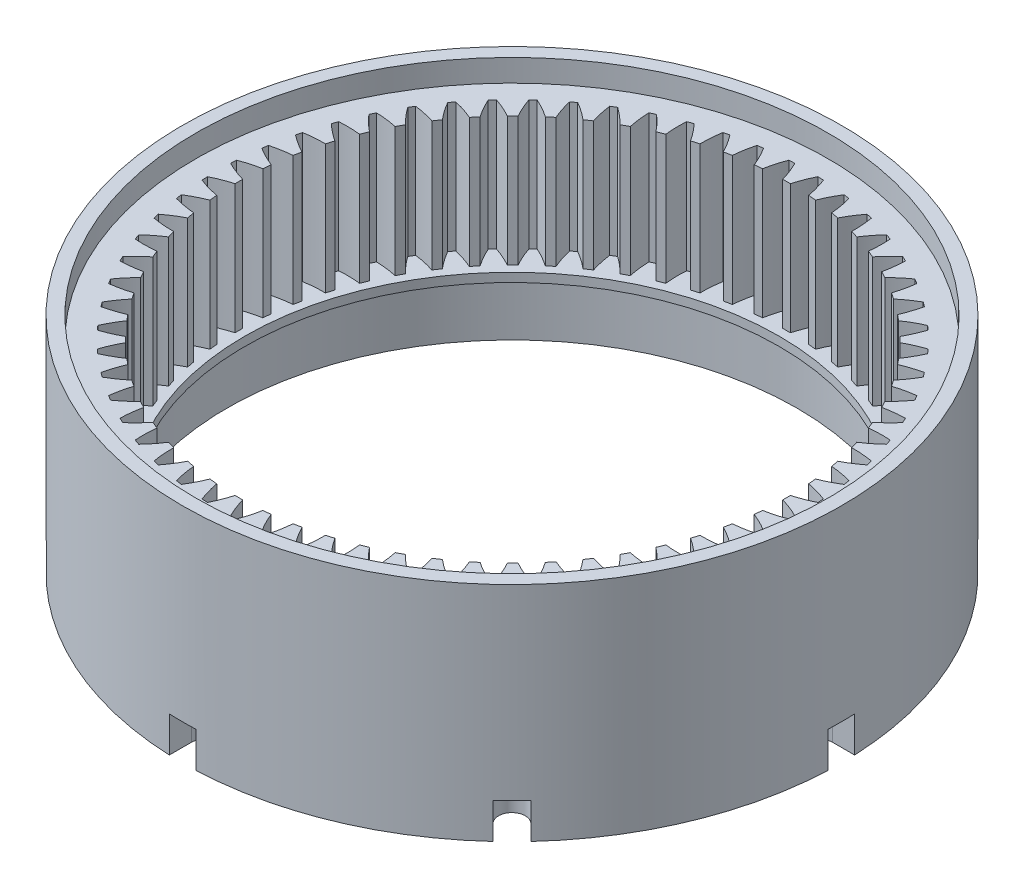
SolidWorks part; units mm, degrees
ref_plane "Front Plane" through (0, 0, 0) normal (0, 0, 1) x (1, 0, 0)
ref_plane "Top Plane" through (0, 0, 0) normal (0, 1, 0) x (1, 0, 0)
ref_plane "Right Plane" through (0, 0, 0) normal (1, 0, 0) x (0, 0, -1)
other "Configuration Table"
sketch "Sketch1" plane through (0, 0, 0) normal (0, 1, 0) x (1, 0, 0)
  circle A0 centre (0, 0) radius 37
  dimension "D1" = 74
extrude "Boss-Extrude1" add sketch "Sketch1" along normal blind 25
sketch "Sketch2" plane through (0, 25, 0) normal (0, 1, 0) x (1, 0, 0)
  circle A0 centre (0, 0) radius 35.5
  dimension "D1" = 71
extrude "Cut-Extrude1" cut sketch "Sketch2" against normal blind 2.5
sketch "Sketch3" plane through (0, 22.5, 0) normal (0, 1, 0) x (1, 0, 0)
  arc A3 (-33.0981, 1.5008) -> (-30.8696, 0.6337) centre (-27.3625, 12.9438) ccw
  arc A4 (-30.8696, 0.6337) -> (-30.8696, -0.2219) centre (-0.1235, 0.2059) ccw
  arc A5 (-30.8696, -0.2219) -> (-33.0981, -1.0891) centre (-27.3625, -12.5321) ccw
  arc A6 (-33.0981, -1.0891) -> (-33.0663, -1.7375) centre (-0.1235, 0.2059) ccw
  arc A7 (-33.0663, -1.7375) -> (-30.7634, -2.382) centre (-28.4798, 10.2126) ccw
  arc A8 (-30.7634, -2.382) -> (-30.6796, -3.2335) centre (-0.1235, 0.2059) ccw
  arc A9 (-30.6796, -3.2335) -> (-32.8124, -4.3149) centre (-25.9828, -15.1406) ccw
  arc A10 (-32.8124, -4.3149) -> (-32.7172, -4.9571) centre (-0.1235, 0.2059) ccw
  arc A11 (-32.7172, -4.9571) -> (-30.3622, -5.3728) centre (-29.3241, 7.385) ccw
  arc A12 (-30.3622, -5.3728) -> (-30.1953, -6.2119) centre (-0.1235, 0.2059) ccw
  arc A13 (-30.1953, -6.2119) -> (-32.2119, -7.4972) centre (-24.354, -17.6013) ccw
  arc A14 (-32.2119, -7.4972) -> (-32.0541, -8.1269) centre (-0.1235, 0.2059) ccw
  arc A15 (-32.0541, -8.1269) -> (-29.6698, -8.3099) centre (-29.8872, 4.4883) ccw
  arc A16 (-29.6698, -8.3099) -> (-29.4215, -9.1286) centre (-0.1235, 0.2059) ccw
  arc A17 (-29.4215, -9.1286) -> (-31.3023, -10.6053) centre (-22.4919, -19.8906) ccw
  arc A18 (-31.3023, -10.6053) -> (-31.0836, -11.2166) centre (-0.1235, 0.2059) ccw
  arc A19 (-31.0836, -11.2166) -> (-28.6929, -11.1649) centre (-30.1636, 1.5503) ccw
  arc A20 (-28.6929, -11.1649) -> (-28.3655, -11.9553) centre (-0.1235, 0.2059) ccw
  arc A21 (-28.3655, -11.9553) -> (-30.0925, -13.6093) centre (-20.4144, -21.9863) ccw
  arc A22 (-30.0925, -13.6093) -> (-29.815, -14.1962) centre (-0.1235, 0.2059) ccw
  arc A23 (-29.815, -14.1962) -> (-27.4408, -13.9104) centre (-30.1508, -1.4006) ccw
  arc A24 (-27.4408, -13.9104) -> (-27.0375, -14.6649) centre (-0.1235, 0.2059) ccw
  arc A25 (-27.0375, -14.6649) -> (-28.5941, -16.4803) centre (-18.1415, -23.8683) ccw
  arc A26 (-28.5941, -16.4803) -> (-28.2603, -17.0371) centre (-0.1235, 0.2059) ccw
  arc A27 (-28.2603, -17.0371) -> (-25.9256, -16.52) centre (-29.8487, -4.336) ccw
  arc A28 (-25.9256, -16.52) -> (-25.4503, -17.2314) centre (-0.1235, 0.2059) ccw
  arc A29 (-25.4503, -17.2314) -> (-26.8215, -19.1905) centre (-15.6951, -25.5185) ccw
  arc A30 (-26.8215, -19.1905) -> (-26.4347, -19.712) centre (-0.1235, 0.2059) ccw
  arc A31 (-26.4347, -19.712) -> (-24.1619, -18.9685) centre (-29.2604, -7.2277) ccw
  arc A32 (-24.1619, -18.9685) -> (-23.6192, -19.6299) centre (-0.1235, 0.2059) ccw
  arc A33 (-23.6192, -19.6299) -> (-24.7917, -21.714) centre (-13.0986, -26.9209) ccw
  arc A34 (-24.7917, -21.714) -> (-24.3557, -22.195) centre (-0.1235, 0.2059) ccw
  arc A35 (-24.3557, -22.195) -> (-22.1667, -21.2323) centre (-28.3915, -10.0479) ccw
  arc A36 (-22.1667, -21.2323) -> (-21.5618, -21.8373) centre (-0.1235, 0.2059) ccw
  arc A37 (-21.5618, -21.8373) -> (-22.5244, -24.0263) centre (-10.3773, -28.062) ccw
  arc A38 (-22.5244, -24.0263) -> (-22.0434, -24.4623) centre (-0.1235, 0.2059) ccw
  arc A39 (-22.0434, -24.4623) -> (-19.9593, -23.2897) centre (-27.2503, -12.7692) ccw
  arc A40 (-19.9593, -23.2897) -> (-19.2979, -23.8325) centre (-0.1235, 0.2059) ccw
  arc A41 (-19.2979, -23.8325) -> (-20.0414, -26.1053) centre (-7.5572, -28.931) ccw
  arc A42 (-20.0414, -26.1053) -> (-19.5199, -26.492) centre (-0.1235, 0.2059) ccw
  arc A43 (-19.5199, -26.492) -> (-17.5608, -25.1208) centre (-25.8479, -15.3656) ccw
  arc A44 (-17.5608, -25.1208) -> (-16.8494, -25.5962) centre (-0.1235, 0.2059) ccw
  arc A45 (-16.8494, -25.5962) -> (-17.3665, -27.9309) centre (-4.6655, -29.5193) ccw
  arc A46 (-17.3665, -27.9309) -> (-16.8097, -28.2647) centre (-0.1235, 0.2059) ccw
  arc A47 (-16.8097, -28.2647) -> (-14.9944, -26.708) centre (-24.1977, -17.8121) ccw
  arc A48 (-14.9944, -26.708) -> (-14.2398, -27.1113) centre (-0.1235, 0.2059) ccw
  arc A49 (-14.2398, -27.1113) -> (-14.5256, -29.4855) centre (-1.73, -29.8213) ccw
  arc A50 (-14.5256, -29.4855) -> (-13.9387, -29.7631) centre (-0.1235, 0.2059) ccw
  arc A51 (-13.9387, -29.7631) -> (-12.2847, -28.036) centre (-22.3158, -20.085) ccw
  arc A52 (-12.2847, -28.036) -> (-11.4943, -28.3634) centre (-0.1235, 0.2059) ccw
  arc A53 (-11.4943, -28.3634) -> (-11.546, -30.7542) centre (1.2209, -29.8342) ccw
  arc A54 (-11.546, -30.7542) -> (-10.9347, -30.9729) centre (-0.1235, 0.2059) ccw
  arc A55 (-10.9347, -30.9729) -> (-9.458, -29.092) centre (-20.22, -22.1625) ccw
  arc A56 (-9.458, -29.092) -> (-8.6393, -29.3404) centre (-0.1235, 0.2059) ccw
  arc A57 (-8.6393, -29.3404) -> (-8.4564, -31.7247) centre (4.1589, -29.5578) ccw
  arc A58 (-8.4564, -31.7247) -> (-7.8266, -31.8825) centre (-0.1235, 0.2059) ccw
  arc A59 (-7.8266, -31.8825) -> (-6.5413, -29.8659) centre (-17.9308, -24.0246) ccw
  arc A60 (-6.5413, -29.8659) -> (-5.7022, -30.0328) centre (-0.1235, 0.2059) ccw
  arc A61 (-5.7022, -30.0328) -> (-5.2865, -32.3877) centre (7.0556, -28.9947) ccw
  arc A62 (-5.2865, -32.3877) -> (-4.6443, -32.483) centre (-0.1235, 0.2059) ccw
  arc A63 (-4.6443, -32.483) -> (-3.5629, -30.3502) centre (-15.47, -25.6533) ccw
  arc A64 (-3.5629, -30.3502) -> (-2.7115, -30.434) centre (-0.1235, 0.2059) ccw
  arc A65 (-2.7115, -30.434) -> (-2.0669, -32.7368) centre (9.8832, -28.1504) ccw
  arc A66 (-2.0669, -32.7368) -> (-1.4185, -32.7687) centre (-0.1235, 0.2059) ccw
  arc A67 (-1.4185, -32.7687) -> (-0.5513, -30.5401) centre (-12.8615, -27.033) ccw
  arc A68 (-0.5513, -30.5401) -> (0.3042, -30.5401) centre (-0.1235, 0.2059) ccw
  arc A69 (0.3042, -30.5401) -> (1.1714, -32.7687) centre (12.6144, -27.033) ccw
  arc A70 (1.1714, -32.7687) -> (1.8198, -32.7368) centre (-0.1235, 0.2059) ccw
  arc A71 (1.8198, -32.7368) -> (2.4644, -30.434) centre (-10.1303, -28.1504) ccw
  arc A72 (2.4644, -30.434) -> (3.3158, -30.3502) centre (-0.1235, 0.2059) ccw
  arc A73 (3.3158, -30.3502) -> (4.3972, -32.483) centre (15.223, -25.6533) ccw
  arc A74 (4.3972, -32.483) -> (5.0394, -32.3877) centre (-0.1235, 0.2059) ccw
  arc A75 (5.0394, -32.3877) -> (5.4552, -30.0328) centre (-7.3027, -28.9947) ccw
  arc A76 (5.4552, -30.0328) -> (6.2943, -29.8659) centre (-0.1235, 0.2059) ccw
  arc A77 (6.2943, -29.8659) -> (7.5795, -31.8825) centre (17.6837, -24.0246) ccw
  arc A78 (7.5795, -31.8825) -> (8.2093, -31.7247) centre (-0.1235, 0.2059) ccw
  arc A79 (8.2093, -31.7247) -> (8.3922, -29.3404) centre (-4.4059, -29.5578) ccw
  arc A80 (8.3922, -29.3404) -> (9.2109, -29.092) centre (-0.1235, 0.2059) ccw
  arc A81 (9.2109, -29.092) -> (10.6877, -30.9729) centre (19.973, -22.1625) ccw
  arc A82 (10.6877, -30.9729) -> (11.2989, -30.7542) centre (-0.1235, 0.2059) ccw
  arc A83 (11.2989, -30.7542) -> (11.2472, -28.3634) centre (-1.468, -29.8342) ccw
  arc A84 (11.2472, -28.3634) -> (12.0377, -28.036) centre (-0.1235, 0.2059) ccw
  arc A85 (12.0377, -28.036) -> (13.6917, -29.7631) centre (22.0687, -20.085) ccw
  arc A86 (13.6917, -29.7631) -> (14.2785, -29.4855) centre (-0.1235, 0.2059) ccw
  arc A87 (14.2785, -29.4855) -> (13.9928, -27.1113) centre (1.4829, -29.8213) ccw
  arc A88 (13.9928, -27.1113) -> (14.7473, -26.708) centre (-0.1235, 0.2059) ccw
  arc A89 (14.7473, -26.708) -> (16.5626, -28.2647) centre (23.9507, -17.8121) ccw
  arc A90 (16.5626, -28.2647) -> (17.1195, -27.9309) centre (-0.1235, 0.2059) ccw
  arc A91 (17.1195, -27.9309) -> (16.6024, -25.5962) centre (4.4184, -29.5193) ccw
  arc A92 (16.6024, -25.5962) -> (17.3137, -25.1208) centre (-0.1235, 0.2059) ccw
  arc A93 (17.3137, -25.1208) -> (19.2729, -26.492) centre (25.6008, -15.3656) ccw
  arc A94 (19.2729, -26.492) -> (19.7943, -26.1053) centre (-0.1235, 0.2059) ccw
  arc A95 (19.7943, -26.1053) -> (19.0509, -23.8325) centre (7.3101, -28.931) ccw
  arc A96 (19.0509, -23.8325) -> (19.7122, -23.2897) centre (-0.1235, 0.2059) ccw
  arc A97 (19.7122, -23.2897) -> (21.7963, -24.4623) centre (27.0032, -12.7692) ccw
  arc A98 (21.7963, -24.4623) -> (22.2774, -24.0263) centre (-0.1235, 0.2059) ccw
  arc A99 (22.2774, -24.0263) -> (21.3147, -21.8373) centre (10.1302, -28.062) ccw
  arc A100 (21.3147, -21.8373) -> (21.9197, -21.2323) centre (-0.1235, 0.2059) ccw
  arc A101 (21.9197, -21.2323) -> (24.1087, -22.195) centre (28.1444, -10.0479) ccw
  arc A102 (24.1087, -22.195) -> (24.5447, -21.714) centre (-0.1235, 0.2059) ccw
  arc A103 (24.5447, -21.714) -> (23.3721, -19.6299) centre (12.8516, -26.9209) ccw
  arc A104 (23.3721, -19.6299) -> (23.9148, -18.9685) centre (-0.1235, 0.2059) ccw
  arc A105 (23.9148, -18.9685) -> (26.1877, -19.712) centre (29.0133, -7.2277) ccw
  arc A106 (26.1877, -19.712) -> (26.5744, -19.1905) centre (-0.1235, 0.2059) ccw
  arc A107 (26.5744, -19.1905) -> (25.2032, -17.2314) centre (15.448, -25.5185) ccw
  arc A108 (25.2032, -17.2314) -> (25.6785, -16.52) centre (-0.1235, 0.2059) ccw
  arc A109 (25.6785, -16.52) -> (28.0133, -17.0371) centre (29.6016, -4.336) ccw
  arc A110 (28.0133, -17.0371) -> (28.347, -16.4803) centre (-0.1235, 0.2059) ccw
  arc A111 (28.347, -16.4803) -> (26.7904, -14.6649) centre (17.8944, -23.8683) ccw
  arc A112 (26.7904, -14.6649) -> (27.1937, -13.9104) centre (-0.1235, 0.2059) ccw
  arc A113 (27.1937, -13.9104) -> (29.5679, -14.1962) centre (29.9037, -1.4006) ccw
  arc A114 (29.5679, -14.1962) -> (29.8455, -13.6093) centre (-0.1235, 0.2059) ccw
  arc A115 (29.8455, -13.6093) -> (28.1184, -11.9553) centre (20.1674, -21.9863) ccw
  arc A116 (28.1184, -11.9553) -> (28.4458, -11.1649) centre (-0.1235, 0.2059) ccw
  arc A117 (28.4458, -11.1649) -> (30.8366, -11.2166) centre (29.9166, 1.5503) ccw
  arc A118 (30.8366, -11.2166) -> (31.0553, -10.6053) centre (-0.1235, 0.2059) ccw
  arc A119 (31.0553, -10.6053) -> (29.1744, -9.1286) centre (22.2449, -19.8906) ccw
  arc A120 (29.1744, -9.1286) -> (29.4228, -8.3099) centre (-0.1235, 0.2059) ccw
  arc A121 (29.4228, -8.3099) -> (31.8071, -8.1269) centre (29.6401, 4.4883) ccw
  arc A122 (31.8071, -8.1269) -> (31.9648, -7.4972) centre (-0.1235, 0.2059) ccw
  arc A123 (31.9648, -7.4972) -> (29.9483, -6.2119) centre (24.107, -17.6013) ccw
  arc A124 (29.9483, -6.2119) -> (30.1152, -5.3728) centre (-0.1235, 0.2059) ccw
  arc A125 (30.1152, -5.3728) -> (32.4701, -4.9571) centre (29.0771, 7.385) ccw
  arc A126 (32.4701, -4.9571) -> (32.5653, -4.3149) centre (-0.1235, 0.2059) ccw
  arc A127 (32.5653, -4.3149) -> (30.4325, -3.2335) centre (25.7357, -15.1406) ccw
  arc A128 (30.4325, -3.2335) -> (30.5164, -2.382) centre (-0.1235, 0.2059) ccw
  arc A129 (30.5164, -2.382) -> (32.8192, -1.7375) centre (28.2328, 10.2126) ccw
  arc A130 (32.8192, -1.7375) -> (32.851, -1.0891) centre (-0.1235, 0.2059) ccw
  arc A131 (32.851, -1.0891) -> (30.6225, -0.2219) centre (27.1154, -12.5321) ccw
  arc A132 (30.6225, -0.2219) -> (30.6225, 0.6337) centre (-0.1235, 0.2059) ccw
  arc A133 (30.6225, 0.6337) -> (32.851, 1.5008) centre (27.1154, 12.9438) ccw
  arc A134 (32.851, 1.5008) -> (32.8192, 2.1493) centre (-0.1235, 0.2059) ccw
  arc A135 (32.8192, 2.1493) -> (30.5164, 2.7938) centre (28.2328, -9.8008) ccw
  arc A136 (30.5164, 2.7938) -> (30.4325, 3.6452) centre (-0.1235, 0.2059) ccw
  arc A137 (30.4325, 3.6452) -> (32.5653, 4.7267) centre (25.7357, 15.5524) ccw
  arc A138 (32.5653, 4.7267) -> (32.4701, 5.3689) centre (-0.1235, 0.2059) ccw
  arc A139 (32.4701, 5.3689) -> (30.1152, 5.7846) centre (29.0771, -6.9732) ccw
  arc A140 (30.1152, 5.7846) -> (29.9483, 6.6237) centre (-0.1235, 0.2059) ccw
  arc A141 (29.9483, 6.6237) -> (31.9648, 7.909) centre (24.107, 18.0131) ccw
  arc A142 (31.9648, 7.909) -> (31.8071, 8.5387) centre (-0.1235, 0.2059) ccw
  arc A143 (31.8071, 8.5387) -> (29.4228, 8.7216) centre (29.6401, -4.0765) ccw
  arc A144 (29.4228, 8.7216) -> (29.1744, 9.5403) centre (-0.1235, 0.2059) ccw
  arc A145 (29.1744, 9.5403) -> (31.0553, 11.0171) centre (22.2449, 20.3024) ccw
  arc A146 (31.0553, 11.0171) -> (30.8366, 11.6283) centre (-0.1235, 0.2059) ccw
  arc A147 (30.8366, 11.6283) -> (28.4458, 11.5767) centre (29.9166, -1.1385) ccw
  arc A148 (28.4458, 11.5767) -> (28.1184, 12.3671) centre (-0.1235, 0.2059) ccw
  arc A149 (28.1184, 12.3671) -> (29.8455, 14.0211) centre (20.1674, 22.3981) ccw
  arc A150 (29.8455, 14.0211) -> (29.5679, 14.608) centre (-0.1235, 0.2059) ccw
  arc A151 (29.5679, 14.608) -> (27.1937, 14.3222) centre (29.9037, 1.8124) ccw
  arc A152 (27.1937, 14.3222) -> (26.7904, 15.0767) centre (-0.1235, 0.2059) ccw
  arc A153 (26.7904, 15.0767) -> (28.347, 16.892) centre (17.8944, 24.2801) ccw
  arc A154 (28.347, 16.892) -> (28.0133, 17.4489) centre (-0.1235, 0.2059) ccw
  arc A155 (28.0133, 17.4489) -> (25.6785, 16.9318) centre (29.6016, 4.7478) ccw
  arc A156 (25.6785, 16.9318) -> (25.2032, 17.6432) centre (-0.1235, 0.2059) ccw
  arc A157 (25.2032, 17.6432) -> (26.5744, 19.6023) centre (15.448, 25.9302) ccw
  arc A158 (26.5744, 19.6023) -> (26.1877, 20.1237) centre (-0.1235, 0.2059) ccw
  arc A159 (26.1877, 20.1237) -> (23.9148, 19.3803) centre (29.0133, 7.6395) ccw
  arc A160 (23.9148, 19.3803) -> (23.3721, 20.0416) centre (-0.1235, 0.2059) ccw
  arc A161 (23.3721, 20.0416) -> (24.5447, 22.1258) centre (12.8516, 27.3327) ccw
  arc A162 (24.5447, 22.1258) -> (24.1087, 22.6068) centre (-0.1235, 0.2059) ccw
  arc A163 (24.1087, 22.6068) -> (21.9197, 21.6441) centre (28.1444, 10.4596) ccw
  arc A164 (21.9197, 21.6441) -> (21.3147, 22.2491) centre (-0.1235, 0.2059) ccw
  arc A165 (21.3147, 22.2491) -> (22.2774, 24.4381) centre (10.1302, 28.4738) ccw
  arc A166 (22.2774, 24.4381) -> (21.7963, 24.8741) centre (-0.1235, 0.2059) ccw
  arc A167 (21.7963, 24.8741) -> (19.7122, 23.7015) centre (27.0032, 13.181) ccw
  arc A168 (19.7122, 23.7015) -> (19.0509, 24.2443) centre (-0.1235, 0.2059) ccw
  arc A169 (19.0509, 24.2443) -> (19.7943, 26.5171) centre (7.3101, 29.3427) ccw
  arc A170 (19.7943, 26.5171) -> (19.2729, 26.9038) centre (-0.1235, 0.2059) ccw
  arc A171 (19.2729, 26.9038) -> (17.3137, 25.5326) centre (25.6008, 15.7774) ccw
  arc A172 (17.3137, 25.5326) -> (16.6024, 26.0079) centre (-0.1235, 0.2059) ccw
  arc A173 (16.6024, 26.0079) -> (17.1195, 28.3427) centre (4.4184, 29.9311) ccw
  arc A174 (17.1195, 28.3427) -> (16.5626, 28.6764) centre (-0.1235, 0.2059) ccw
  arc A175 (16.5626, 28.6764) -> (14.7473, 27.1198) centre (23.9507, 18.2239) ccw
  arc A176 (14.7473, 27.1198) -> (13.9928, 27.5231) centre (-0.1235, 0.2059) ccw
  arc A177 (13.9928, 27.5231) -> (14.2785, 29.8973) centre (1.4829, 30.2331) ccw
  arc A178 (14.2785, 29.8973) -> (13.6917, 30.1749) centre (-0.1235, 0.2059) ccw
  arc A179 (13.6917, 30.1749) -> (12.0377, 28.4478) centre (22.0687, 20.4968) ccw
  arc A180 (12.0377, 28.4478) -> (11.2472, 28.7752) centre (-0.1235, 0.2059) ccw
  arc A181 (11.2472, 28.7752) -> (11.2989, 31.166) centre (-1.468, 30.246) ccw
  arc A182 (11.2989, 31.166) -> (10.6877, 31.3847) centre (-0.1235, 0.2059) ccw
  arc A183 (10.6877, 31.3847) -> (9.2109, 29.5038) centre (19.973, 22.5743) ccw
  arc A184 (9.2109, 29.5038) -> (8.3922, 29.7522) centre (-0.1235, 0.2059) ccw
  arc A185 (8.3922, 29.7522) -> (8.2093, 32.1365) centre (-4.4059, 29.9696) ccw
  arc A186 (8.2093, 32.1365) -> (7.5795, 32.2942) centre (-0.1235, 0.2059) ccw
  arc A187 (7.5795, 32.2942) -> (6.2943, 30.2777) centre (17.6837, 24.4364) ccw
  arc A188 (6.2943, 30.2777) -> (5.4552, 30.4446) centre (-0.1235, 0.2059) ccw
  arc A189 (5.4552, 30.4446) -> (5.0394, 32.7995) centre (-7.3027, 29.4065) ccw
  arc A190 (5.0394, 32.7995) -> (4.3972, 32.8948) centre (-0.1235, 0.2059) ccw
  arc A191 (4.3972, 32.8948) -> (3.3158, 30.7619) centre (15.223, 26.0651) ccw
  arc A192 (3.3158, 30.7619) -> (2.4644, 30.8458) centre (-0.1235, 0.2059) ccw
  arc A193 (2.4644, 30.8458) -> (1.8198, 33.1486) centre (-10.1303, 28.5622) ccw
  arc A194 (1.8198, 33.1486) -> (1.1714, 33.1805) centre (-0.1235, 0.2059) ccw
  arc A195 (1.1714, 33.1805) -> (0.3042, 30.9519) centre (12.6144, 27.4448) ccw
  arc A196 (0.3042, 30.9519) -> (-0.5513, 30.9519) centre (-0.1235, 0.2059) ccw
  arc A197 (-0.5513, 30.9519) -> (-1.4185, 33.1805) centre (-12.8615, 27.4448) ccw
  arc A198 (-1.4185, 33.1805) -> (-2.0669, 33.1486) centre (-0.1235, 0.2059) ccw
  arc A199 (-2.0669, 33.1486) -> (-2.7115, 30.8458) centre (9.8832, 28.5622) ccw
  arc A200 (-2.7115, 30.8458) -> (-3.5629, 30.7619) centre (-0.1235, 0.2059) ccw
  arc A201 (-3.5629, 30.7619) -> (-4.6443, 32.8948) centre (-15.47, 26.0651) ccw
  arc A202 (-4.6443, 32.8948) -> (-5.2865, 32.7995) centre (-0.1235, 0.2059) ccw
  arc A203 (-5.2865, 32.7995) -> (-5.7022, 30.4446) centre (7.0556, 29.4065) ccw
  arc A204 (-5.7022, 30.4446) -> (-6.5413, 30.2777) centre (-0.1235, 0.2059) ccw
  arc A205 (-6.5413, 30.2777) -> (-7.8266, 32.2942) centre (-17.9308, 24.4364) ccw
  arc A206 (-7.8266, 32.2942) -> (-8.4564, 32.1365) centre (-0.1235, 0.2059) ccw
  arc A207 (-8.4564, 32.1365) -> (-8.6393, 29.7522) centre (4.1589, 29.9696) ccw
  arc A208 (-8.6393, 29.7522) -> (-9.458, 29.5038) centre (-0.1235, 0.2059) ccw
  arc A209 (-9.458, 29.5038) -> (-10.9347, 31.3847) centre (-20.22, 22.5743) ccw
  arc A210 (-10.9347, 31.3847) -> (-11.546, 31.166) centre (-0.1235, 0.2059) ccw
  arc A211 (-11.546, 31.166) -> (-11.4943, 28.7752) centre (1.2209, 30.246) ccw
  arc A212 (-11.4943, 28.7752) -> (-12.2847, 28.4478) centre (-0.1235, 0.2059) ccw
  arc A213 (-12.2847, 28.4478) -> (-13.9387, 30.1749) centre (-22.3158, 20.4968) ccw
  arc A214 (-13.9387, 30.1749) -> (-14.5256, 29.8973) centre (-0.1235, 0.2059) ccw
  arc A215 (-14.5256, 29.8973) -> (-14.2398, 27.5231) centre (-1.73, 30.2331) ccw
  arc A216 (-14.2398, 27.5231) -> (-14.9944, 27.1198) centre (-0.1235, 0.2059) ccw
  arc A217 (-14.9944, 27.1198) -> (-16.8097, 28.6764) centre (-24.1977, 18.2239) ccw
  arc A218 (-16.8097, 28.6764) -> (-17.3665, 28.3427) centre (-0.1235, 0.2059) ccw
  arc A219 (-17.3665, 28.3427) -> (-16.8494, 26.0079) centre (-4.6655, 29.9311) ccw
  arc A220 (-16.8494, 26.0079) -> (-17.5608, 25.5326) centre (-0.1235, 0.2059) ccw
  arc A221 (-17.5608, 25.5326) -> (-19.5199, 26.9038) centre (-25.8479, 15.7774) ccw
  arc A222 (-19.5199, 26.9038) -> (-20.0414, 26.5171) centre (-0.1235, 0.2059) ccw
  arc A223 (-20.0414, 26.5171) -> (-19.2979, 24.2443) centre (-7.5572, 29.3427) ccw
  arc A224 (-19.2979, 24.2443) -> (-19.9593, 23.7015) centre (-0.1235, 0.2059) ccw
  arc A225 (-19.9593, 23.7015) -> (-22.0434, 24.8741) centre (-27.2503, 13.181) ccw
  arc A226 (-22.0434, 24.8741) -> (-22.5244, 24.4381) centre (-0.1235, 0.2059) ccw
  arc A227 (-22.5244, 24.4381) -> (-21.5618, 22.2491) centre (-10.3773, 28.4738) ccw
  arc A228 (-21.5618, 22.2491) -> (-22.1667, 21.6441) centre (-0.1235, 0.2059) ccw
  arc A229 (-22.1667, 21.6441) -> (-24.3557, 22.6068) centre (-28.3915, 10.4596) ccw
  arc A230 (-24.3557, 22.6068) -> (-24.7917, 22.1258) centre (-0.1235, 0.2059) ccw
  arc A231 (-24.7917, 22.1258) -> (-23.6192, 20.0416) centre (-13.0986, 27.3327) ccw
  arc A232 (-23.6192, 20.0416) -> (-24.1619, 19.3803) centre (-0.1235, 0.2059) ccw
  arc A233 (-24.1619, 19.3803) -> (-26.4347, 20.1237) centre (-29.2604, 7.6395) ccw
  arc A234 (-26.4347, 20.1237) -> (-26.8215, 19.6023) centre (-0.1235, 0.2059) ccw
  arc A235 (-26.8215, 19.6023) -> (-25.4503, 17.6432) centre (-15.6951, 25.9302) ccw
  arc A236 (-25.4503, 17.6432) -> (-25.9256, 16.9318) centre (-0.1235, 0.2059) ccw
  arc A237 (-25.9256, 16.9318) -> (-28.2603, 17.4489) centre (-29.8487, 4.7478) ccw
  arc A238 (-28.2603, 17.4489) -> (-28.5941, 16.892) centre (-0.1235, 0.2059) ccw
  arc A239 (-28.5941, 16.892) -> (-27.0375, 15.0767) centre (-18.1415, 24.2801) ccw
  arc A240 (-27.0375, 15.0767) -> (-27.4408, 14.3222) centre (-0.1235, 0.2059) ccw
  arc A241 (-27.4408, 14.3222) -> (-29.815, 14.608) centre (-30.1508, 1.8124) ccw
  arc A242 (-29.815, 14.608) -> (-30.0925, 14.0211) centre (-0.1235, 0.2059) ccw
  arc A243 (-30.0925, 14.0211) -> (-28.3655, 12.3671) centre (-20.4144, 22.3981) ccw
  arc A244 (-28.3655, 12.3671) -> (-28.6929, 11.5767) centre (-0.1235, 0.2059) ccw
  arc A245 (-28.6929, 11.5767) -> (-31.0836, 11.6283) centre (-30.1636, -1.1385) ccw
  arc A246 (-31.0836, 11.6283) -> (-31.3023, 11.0171) centre (-0.1235, 0.2059) ccw
  arc A247 (-31.3023, 11.0171) -> (-29.4215, 9.5403) centre (-22.4919, 20.3024) ccw
  arc A248 (-29.4215, 9.5403) -> (-29.6698, 8.7216) centre (-0.1235, 0.2059) ccw
  arc A249 (-29.6698, 8.7216) -> (-32.0541, 8.5387) centre (-29.8872, -4.0765) ccw
  arc A250 (-32.0541, 8.5387) -> (-32.2119, 7.909) centre (-0.1235, 0.2059) ccw
  arc A251 (-32.2119, 7.909) -> (-30.1953, 6.6237) centre (-24.354, 18.0131) ccw
  arc A252 (-30.1953, 6.6237) -> (-30.3622, 5.7846) centre (-0.1235, 0.2059) ccw
  arc A253 (-30.3622, 5.7846) -> (-32.7172, 5.3689) centre (-29.3241, -6.9732) ccw
  arc A254 (-32.7172, 5.3689) -> (-32.8124, 4.7267) centre (-0.1235, 0.2059) ccw
  arc A255 (-32.8124, 4.7267) -> (-30.6796, 3.6452) centre (-25.9828, 15.5524) ccw
  arc A256 (-30.6796, 3.6452) -> (-30.7634, 2.7938) centre (-0.1235, 0.2059) ccw
  arc A257 (-30.7634, 2.7938) -> (-33.0663, 2.1493) centre (-28.4798, -9.8008) ccw
  arc A258 (-33.0663, 2.1493) -> (-33.0981, 1.5008) centre (-0.1235, 0.2059) ccw
extrude "Cut-Extrude2" cut sketch "Sketch3" against normal blind 14.5
sketch "Sketch4" plane through (0, 0, 0) normal (0, -1, 0) x (1, 0, 0)
  circle A0 centre (0, 0) radius 30
  dimension "D1" = 60
extrude "Cut-Extrude3" cut sketch "Sketch4" against normal blind 62.5
sketch "Sketch5" plane through (0, 0, 0) normal (0, -1, 0) x (1, 0, 0)
  circle A0 centre (0, 0) radius 32
  dimension "D1" = 64
extrude "Cut-Extrude4" cut sketch "Sketch5" against normal blind 7
sketch "Sketch6" plane through (0, 0, 0) normal (0, -1, 0) x (1, 0, 0)
  line L0 (22.6274, 26.163) -> (23.6266, 27.1622)
  line L1 (-2.5, 34.5) -> (-2.5, 35.9131)
  line L3 (2.5, 35.9131) -> (2.5, 34.5)
  line L5 (27.1622, 23.6266) -> (26.163, 22.6274)
  line L7 (34.5, 2.5) -> (35.9131, 2.5)
  line L8 (35.9131, -2.5) -> (34.5, -2.5)
  line L10 (26.163, -22.6274) -> (27.1622, -23.6266)
  line L11 (23.6266, -27.1622) -> (22.6274, -26.163)
  line L13 (2.5, -34.5) -> (2.5, -35.9131)
  line L14 (-2.5, -35.9131) -> (-2.5, -34.5)
  line L16 (-22.6274, -26.163) -> (-23.6266, -27.1622)
  line L17 (-27.1622, -23.6266) -> (-26.163, -22.6274)
  line L19 (-34.5, -2.5) -> (-35.9131, -2.5)
  line L20 (-35.9131, 2.5) -> (-34.5, 2.5)
  line L22 (-26.163, 22.6274) -> (-27.1622, 23.6266)
  line L23 (-23.6266, 27.1622) -> (-22.6274, 26.163)
  arc A0 (-35.9131, -2.5) -> (-27.1622, -23.6266) centre (0, 0) ccw
  arc A1 (-32.942, -1.9552) -> (-24.6761, -21.911) centre (0, 0) ccw
  arc A3 (1.9552, 32.942) -> (2.5, 34.5) centre (0, 34.5) ccw
  arc A4 (-2.5, 34.5) -> (-1.9552, 32.942) centre (0, 34.5) ccw
  arc A5 (22.6274, 26.163) -> (21.911, 24.6761) centre (24.3952, 24.3952) ccw
  arc A6 (24.6761, 21.911) -> (26.163, 22.6274) centre (24.3952, 24.3952) ccw
  arc A7 (34.5, 2.5) -> (32.942, 1.9552) centre (34.5, 0) ccw
  arc A8 (32.942, -1.9552) -> (34.5, -2.5) centre (34.5, 0) ccw
  arc A9 (26.163, -22.6274) -> (24.6761, -21.911) centre (24.3952, -24.3952) ccw
  arc A10 (21.911, -24.6761) -> (22.6274, -26.163) centre (24.3952, -24.3952) ccw
  arc A11 (2.5, -34.5) -> (1.9552, -32.942) centre (0, -34.5) ccw
  arc A12 (-1.9552, -32.942) -> (-2.5, -34.5) centre (0, -34.5) ccw
  arc A13 (-22.6274, -26.163) -> (-21.911, -24.6761) centre (-24.3952, -24.3952) ccw
  arc A14 (-24.6761, -21.911) -> (-26.163, -22.6274) centre (-24.3952, -24.3952) ccw
  arc A15 (-34.5, -2.5) -> (-32.942, -1.9552) centre (-34.5, 0) ccw
  arc A16 (-32.942, 1.9552) -> (-34.5, 2.5) centre (-34.5, 0) ccw
  arc A17 (-26.163, 22.6274) -> (-24.6761, 21.911) centre (-24.3952, 24.3952) ccw
  arc A18 (-21.911, 24.6761) -> (-22.6274, 26.163) centre (-24.3952, 24.3952) ccw
  arc A19 (-24.6761, 21.911) -> (-32.942, 1.9552) centre (0, 0) ccw
  arc A20 (-27.1622, 23.6266) -> (-35.9131, 2.5) centre (0, 0) ccw
  arc A21 (-2.5, 35.9131) -> (-23.6266, 27.1622) centre (0, 0) ccw
  arc A22 (-1.9552, 32.942) -> (-21.911, 24.6761) centre (0, 0) ccw
  arc A23 (23.6266, 27.1622) -> (2.5, 35.9131) centre (0, 0) ccw
  arc A24 (21.911, 24.6761) -> (1.9552, 32.942) centre (0, 0) ccw
  arc A25 (35.9131, 2.5) -> (27.1622, 23.6266) centre (0, 0) ccw
  arc A26 (32.942, 1.9552) -> (24.6761, 21.911) centre (0, 0) ccw
  arc A27 (27.1622, -23.6266) -> (35.9131, -2.5) centre (0, 0) ccw
  arc A28 (24.6761, -21.911) -> (32.942, -1.9552) centre (0, 0) ccw
  arc A29 (1.9552, -32.942) -> (21.911, -24.6761) centre (0, 0) ccw
  arc A30 (2.5, -35.9131) -> (23.6266, -27.1622) centre (0, 0) ccw
  arc A31 (-21.911, -24.6761) -> (-1.9552, -32.942) centre (0, 0) ccw
  arc A32 (-23.6266, -27.1622) -> (-2.5, -35.9131) centre (0, 0) ccw
  point P65 (0, 0)
  dimension "D1" = 66
  dimension "D2" = 72
  dimension "D3" = 34.5
  dimension "D5" = 8
  dimension "D4" = 5
extrude "Cut-Extrude5" cut sketch "Sketch6" against normal blind 6
sketch "Sketch7" plane through (0, 0, 0) normal (0, -1, 0) x (1, 0, 0)
  line L0 (-1.5, 34.5) -> (-1.5, 38.934)
  line L1 (-1.5, 38.934) -> (1.5, 38.934)
  line L2 (1.5, 38.934) -> (1.5, 34.5)
  arc A0 (-1.5, 34.5) -> (1.5, 34.5) centre (0, 34.5) ccw
  dimension "D1" = 3
extrude "Cut-Extrude6" cut sketch "Sketch7" against normal blind 4
pattern_circular "CirPattern1" count 8 over 360 about axis through (0, 0, 0) along (0, 1, 0) of "Cut-Extrude6"
